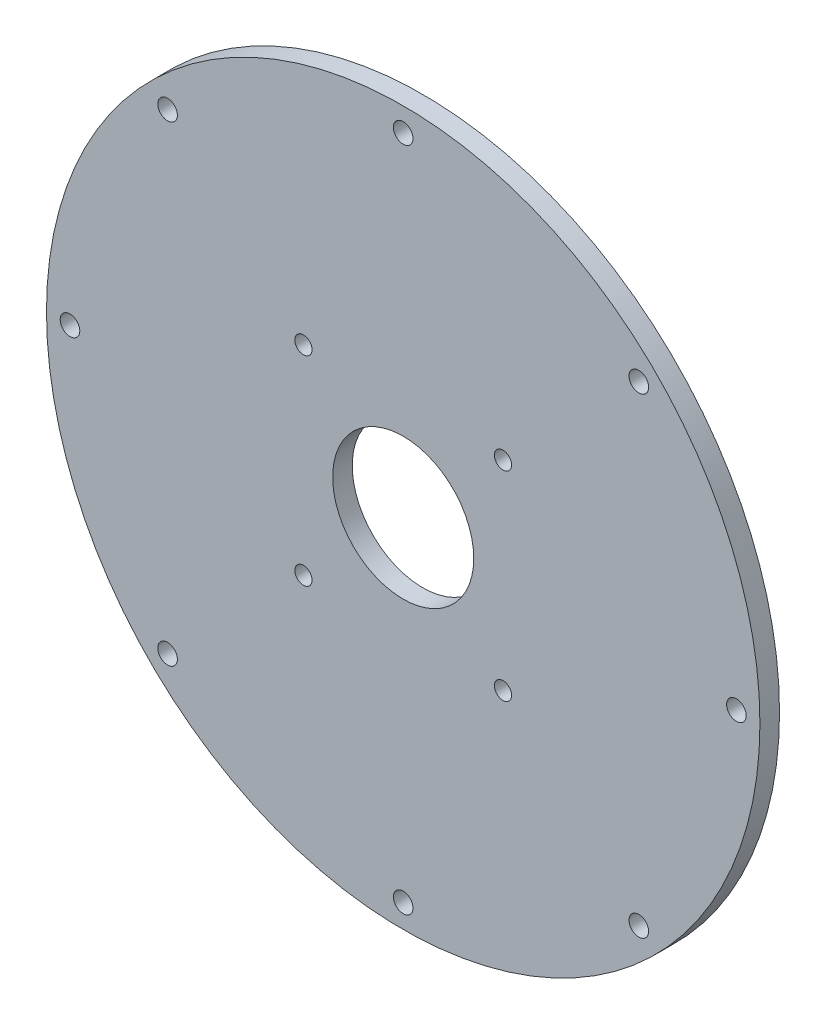
from build123d import *

# Parameters (mm, degrees)
SKETCH_1_R               = 91
SKETCH_1_R_2             = 18
EXTRUDE_1_DEPTH          = 2.5
SKETCH_2_R               = 2.5
CUT_EXTRUDE_1_DEPTH      = 5
PATTERN_CIRCULAR_1_COUNT = 8
SKETCH_3_R               = 2.2
CUT_EXTRUDE_2_DEPTH      = 10
PATTERN_CIRCULAR_2_COUNT = 4


with BuildPart() as part:
    # 草图1 → 凸台-拉伸1 (new, symmetric)
    with BuildSketch(Plane.XY):
        Circle(SKETCH_1_R)
        Circle(SKETCH_1_R_2, mode=Mode.SUBTRACT)
    extrude(amount=EXTRUDE_1_DEPTH, both=True)

    # 草图2 → 切除-拉伸1 (cut)
    with BuildSketch(Plane.XY.offset(2.5)):
        with Locations((0, 85)):
            Circle(SKETCH_2_R)
    cut_extrude_1 = extrude(amount=-CUT_EXTRUDE_1_DEPTH, mode=Mode.SUBTRACT)

    # 阵列(圆周)1: 切除-拉伸1 ×8 about axis
    pattern_circular_1_axis = Axis((0, 0, 0), (0, 0, 1))
    for i in range(1, PATTERN_CIRCULAR_1_COUNT):
        add(cut_extrude_1.rotate(pattern_circular_1_axis, i * 360 / PATTERN_CIRCULAR_1_COUNT), mode=Mode.SUBTRACT)

    # 草图3 → 切除-拉伸2 (cut)
    with BuildSketch(Plane(origin=(0, 0, -2.5), x_dir=(-1, 0, 0), z_dir=(0, 0, -1))):
        with Locations((25.455844123, 25.455844123)):
            Circle(SKETCH_3_R)
    cut_extrude_2 = extrude(amount=-CUT_EXTRUDE_2_DEPTH, mode=Mode.SUBTRACT)

    # 阵列(圆周)2: 切除-拉伸2 ×4 about axis
    pattern_circular_2_axis = Axis((0, 0, 0), (0, 0, 1))
    for i in range(1, PATTERN_CIRCULAR_2_COUNT):
        add(cut_extrude_2.rotate(pattern_circular_2_axis, i * 360 / PATTERN_CIRCULAR_2_COUNT), mode=Mode.SUBTRACT)


solid = part.part
